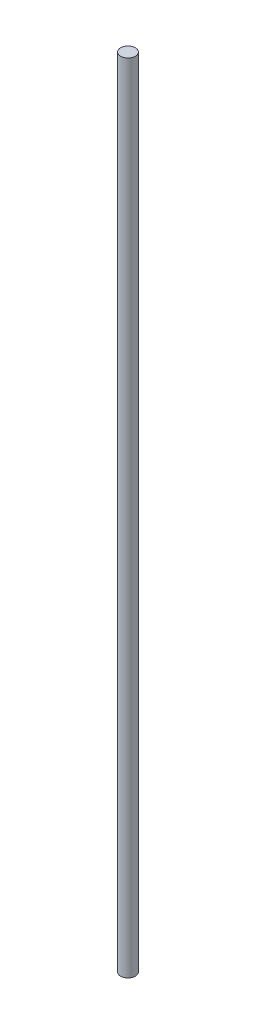
from build123d import *

# Parameters (mm, degrees)
SKETCH1_R           = 1.5
BOSS_EXTRUDE1_DEPTH = 162


with BuildPart() as part:
    # Sketch1 → Boss-Extrude1 (new body)
    with BuildSketch(Plane(origin=(0, 0, 0), x_dir=(1, 0, 0), z_dir=(0, 1, 0))):
        with Locations(Location((0, 0, 0), (0, 0, 270))):
            Circle(SKETCH1_R)
    extrude(amount=BOSS_EXTRUDE1_DEPTH)


solid = part.part
